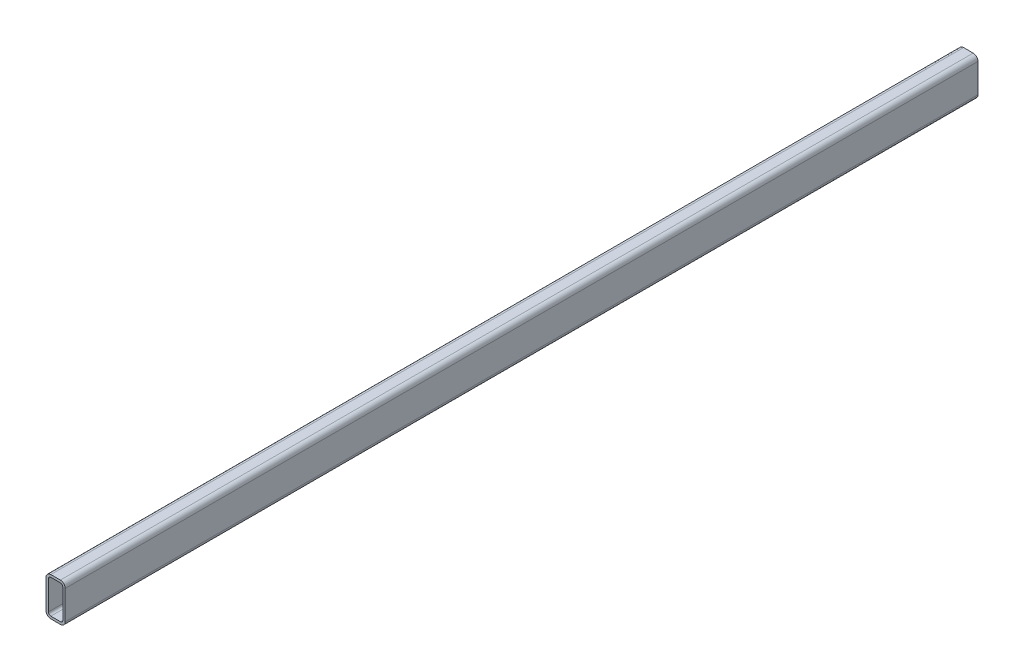
from build123d import *

# Parameters (mm, degrees)
BOSS_EXTRUDE1_DEPTH = 1900


with BuildPart() as part:
    # Sketch1 → Boss-Extrude1 (new body)
    with BuildSketch(Plane.XY):
        with BuildLine():
            Line((-10, -40), (10, -40))
            ThreePointArc((10, -40), (17.071067812, -37.071067812), (20, -30))
            Line((20, -30), (20, 30))
            ThreePointArc((20, 30), (17.071067812, 37.071067812), (10, 40))
            Line((10, 40), (-10, 40))
            ThreePointArc((-10, 40), (-17.071067812, 37.071067812), (-20, 30))
            Line((-20, 30), (-20, -30))
            ThreePointArc((-20, -30), (-17.071067812, -37.071067812), (-10, -40))
        make_face()
        with BuildLine():
            Line((-10, -35), (10, -35))
            ThreePointArc((10, -35), (13.535533906, -33.535533906), (15, -30))
            Line((15, -30), (15, 30))
            ThreePointArc((15, 30), (13.535533906, 33.535533906), (10, 35))
            Line((10, 35), (-10, 35))
            ThreePointArc((-10, 35), (-13.535533906, 33.535533906), (-15, 30))
            Line((-15, 30), (-15, -30))
            ThreePointArc((-15, -30), (-13.535533906, -33.535533906), (-10, -35))
        make_face(mode=Mode.SUBTRACT)
    extrude(amount=BOSS_EXTRUDE1_DEPTH)


solid = part.part
